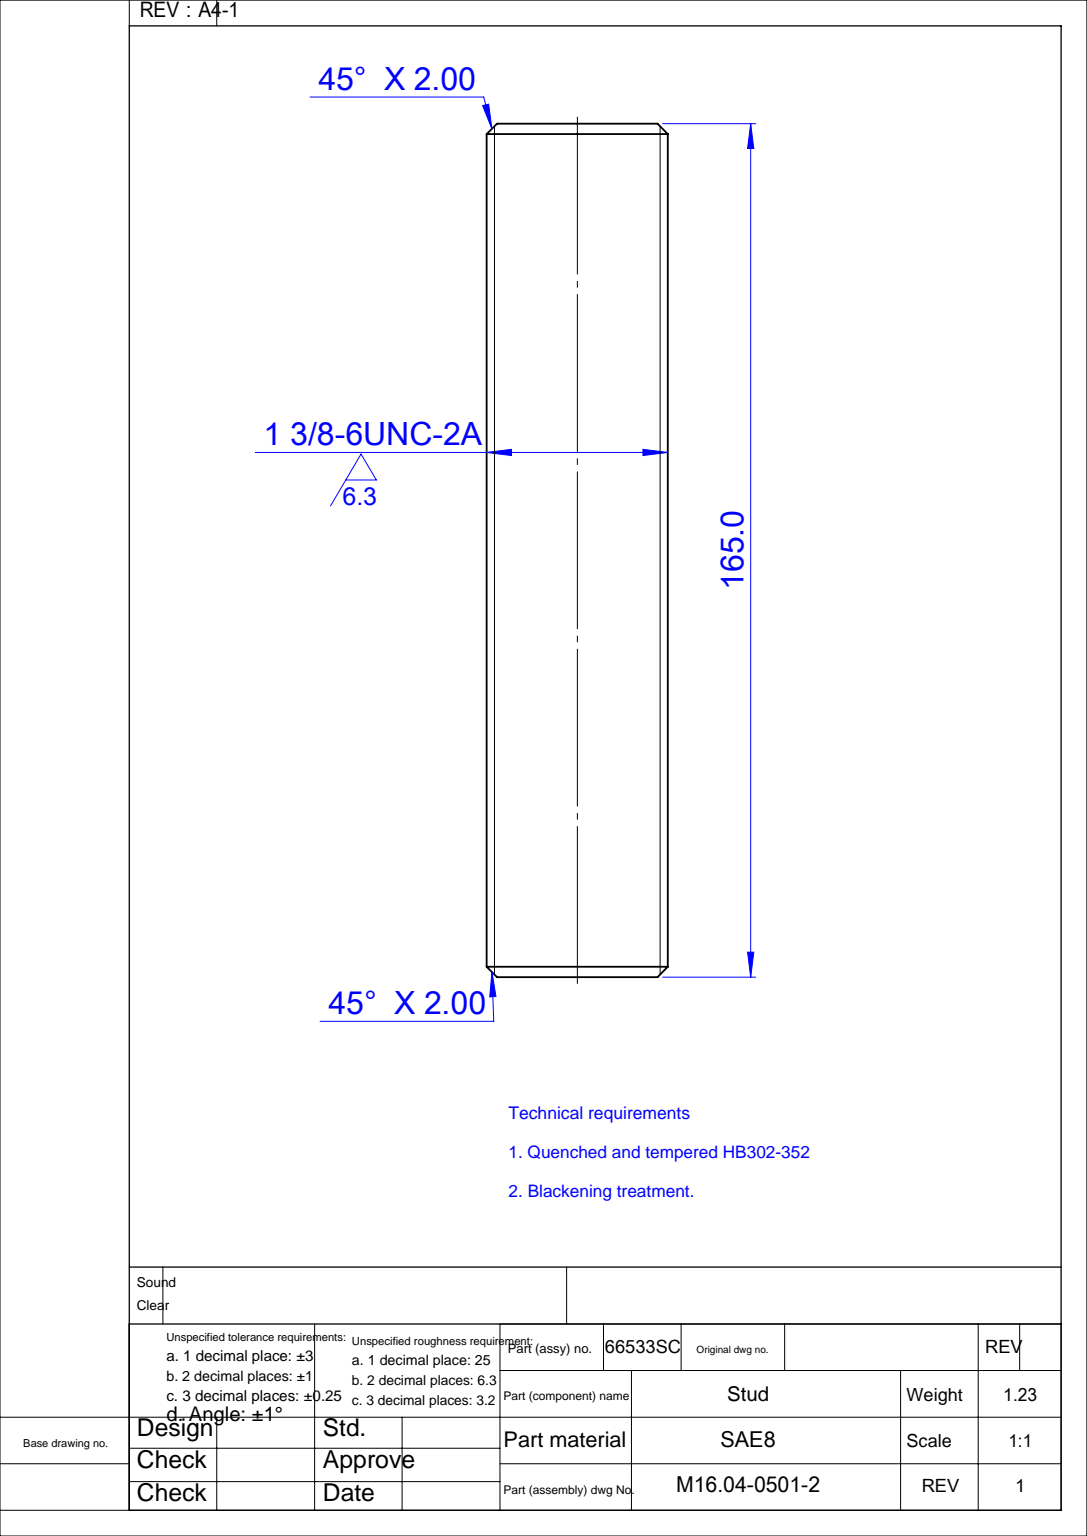
from build123d import *

# Parameters (mm, degrees)
SKETCH1_W     = 17.5
SKETCH1_H     = 165
CHAMFER1_SIZE = 2


with BuildPart() as part:
    # Sketch1 → Revolve1 (revolve)
    with BuildSketch(Plane.XY, mode=Mode.PRIVATE) as revolve1_sk:
        with Locations((-8.75, 82.5)):
            Rectangle(SKETCH1_W, SKETCH1_H)
    revolve(revolve1_sk.sketch.rotate(Axis((0, 158.86069982, 0), (0, -1, 0)), 270), axis=Axis((0, 158.86069982, 0), (0, -1, 0)))

    # Chamfer1
    chamfer1_edges = [part.edges().sort_by_distance(p)[0] for p in [
        (0, 0, -17.5),
        (0, 165, -17.5),
    ]]
    chamfer(chamfer1_edges, length=CHAMFER1_SIZE)


solid = part.part
